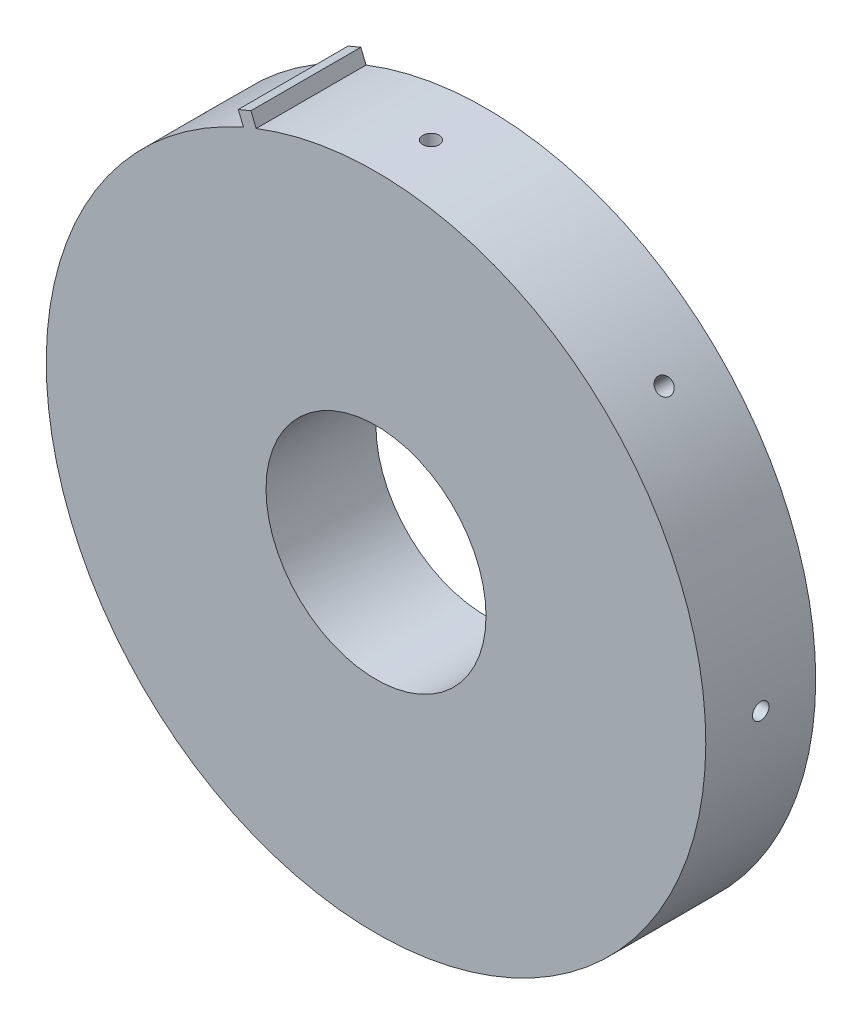
from build123d import *

# Parameters (mm, degrees)
SKETCH1_R           = 120
SKETCH1_R_2         = 40.03000000000001
BOSS_EXTRUDE1_DEPTH = 40
SKETCH2_R           = 2.654999999999998
CUT_EXTRUDE1_DEPTH  = 10
SKETCH3_R           = 3.000000000000001
CUT_EXTRUDE3_DEPTH  = 10
SKETCH6_R           = 3.000000000000003
CUT_EXTRUDE4_DEPTH  = 50.7
CIRPATTERN1_COUNT   = 8
BOSS_EXTRUDE2_DEPTH = 40


with BuildPart() as part:
    # Sketch1 → Boss-Extrude1 (new body)
    with BuildSketch(Plane.XY):
        Circle(SKETCH1_R)
        Circle(SKETCH1_R_2, mode=Mode.SUBTRACT)
    extrude(amount=BOSS_EXTRUDE1_DEPTH)

    # Sketch2 → Cut-Extrude1 (cut)
    with BuildSketch(Plane(origin=(0, 0, 0), x_dir=(-1, 0, 0), z_dir=(0, 0, -1))):
        with Locations((0, 69.3)):
            Circle(SKETCH2_R)
    cut_extrude1 = extrude(amount=-CUT_EXTRUDE1_DEPTH, mode=Mode.SUBTRACT)

    # Sketch3 → Cut-Extrude3 (cut)
    with BuildSketch(Plane(origin=(0, 0, 10), x_dir=(-1, 0, 0), z_dir=(0, 0, -1))):
        with Locations((0, 69.3)):
            Circle(SKETCH3_R)
    cut_extrude3 = extrude(amount=-CUT_EXTRUDE3_DEPTH, mode=Mode.SUBTRACT)

    # Sketch5 → Cut-Revolve1 (revolve, cut)
    with BuildSketch(Plane(origin=(0, 0, 20), x_dir=(-1, 0, 0), z_dir=(0, 0, -1))):
        with BuildLine():
            Line((0, 72.3), (0, 66.3))
            ThreePointArc((0, 66.3), (3, 69.3), (0, 72.3))
        make_face()
    cut_revolve1 = revolve(axis=Axis((0, 72.3, 20), (0, -1, 0)), mode=Mode.SUBTRACT)

    # Sketch6 → Cut-Extrude4 (cut)
    with BuildSketch(Plane(origin=(0, 120, 0), x_dir=(1, 0, 0), z_dir=(0, 1, 0))):
        with Locations(Location((0, -20, 0), (0, 0, 270))):
            Circle(SKETCH6_R)
    cut_extrude4 = extrude(amount=-CUT_EXTRUDE4_DEPTH, mode=Mode.SUBTRACT)

    # CirPattern1: Cut-Extrude1, Cut-Extrude3, Cut-Revolve1, Cut-Extrude4 ×8 about axis
    cirpattern1_axis = Axis((-6.08e-14, 1.3e-16, 0), (0, 0, 1))
    add([cut_extrude1.rotate(cirpattern1_axis, i * 360 / CIRPATTERN1_COUNT) for i in range(1, CIRPATTERN1_COUNT)], mode=Mode.SUBTRACT)
    add([cut_extrude3.rotate(cirpattern1_axis, i * 360 / CIRPATTERN1_COUNT) for i in range(1, CIRPATTERN1_COUNT)], mode=Mode.SUBTRACT)
    add([cut_revolve1.rotate(cirpattern1_axis, i * 360 / CIRPATTERN1_COUNT) for i in range(1, CIRPATTERN1_COUNT)], mode=Mode.SUBTRACT)
    add([cut_extrude4.rotate(cirpattern1_axis, i * 360 / CIRPATTERN1_COUNT) for i in range(1, CIRPATTERN1_COUNT)], mode=Mode.SUBTRACT)

    # Sketch7 → Boss-Extrude2 (add)
    with BuildSketch(Plane(origin=(0, 0, 0), x_dir=(-1, 0, 0), z_dir=(0, 0, -1))):
        Polygon((45.525730214358006, 116.44165014482351), (50.14512787691445, 114.52823298299805), (47.7461408529735, 108.73656597384273), (43.126743190417045, 110.6499831356682), align=None)
    extrude(amount=-BOSS_EXTRUDE2_DEPTH)


solid = part.part
